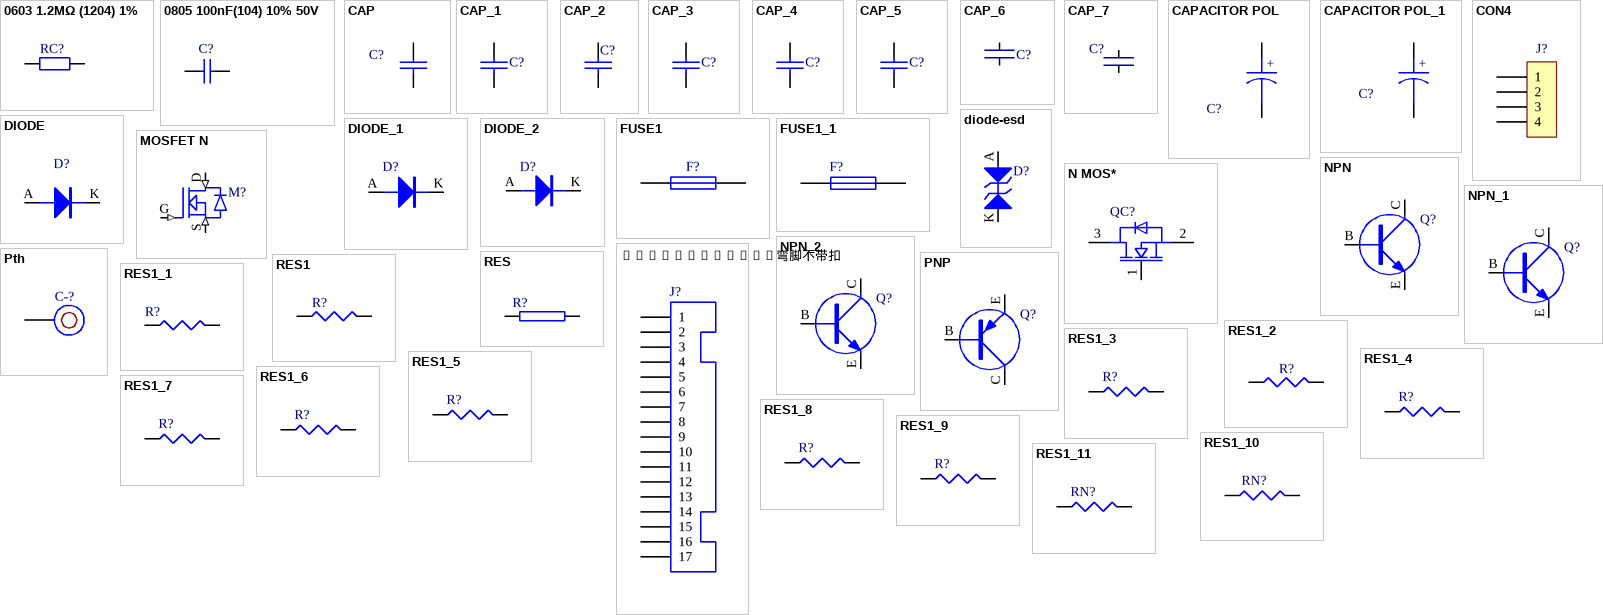
[diagram p0: symbols 0603 1.2MΩ (1204) 1% to RES1_11]
# Altium schematic symbol library MISC86327.SCHLIB: 73 symbols
Pins are listed as number, name and electrical type; pins without a type are passive.


## 0603 1.2MΩ (1204) 1%
designator RC?
chip resistor
footprint RES0603 (CAP0402)
footprint R0603
footprint R0603A (chip resistor)
pins: 1, 2
2 alternate drawings of the same symbol

## 0805 100nF(104) 10% 50V
designator C?
chip capacitor
footprint CAP0603 (CAP0402)
footprint C0603
footprint C0603A (chip capacitor)
pins: 1, 2
2 alternate drawings of the same symbol

## CAP
designator C?
Capacitor
footprint C0603
footprint C0603M (chip capacitor)
pins: 1, 2
2 alternate drawings of the same symbol

## CAP_1
designator C?
Capacitor
footprint C0805
pins: 1, 2
2 alternate drawings of the same symbol

## CAP_2
designator C?
Capacitor
footprint C0603
footprint C0603M (chip capacitor)
pins: 1, 2
2 alternate drawings of the same symbol

## CAP_3
designator C?
Capacitor
footprint C0603
footprint C0805
pins: 1, 2
2 alternate drawings of the same symbol

## CAP_4
designator C?
Capacitor
footprint C0603
footprint C0603M (chip capacitor)
pins: 1, 2
2 alternate drawings of the same symbol

## CAP_5
designator C?
Capacitor
footprint C0603
footprint C0603M (chip capacitor)
pins: 1, 2
2 alternate drawings of the same symbol

## CAP_6
designator C?
CAP
footprint CAP0603 (CAP0402)
footprint C0603
footprint C0603M (chip capacitor)
pins: 1, 2

## CAP_7
designator C?
CAP
footprint CAP0603 (CAP0402)
footprint C0603
footprint C0603M (chip capacitor)
pins: 1, 2

## CAPACITOR POL
designator C?
Capacitor
footprint C0805
pins: 1, 2

## CAPACITOR POL_1
designator C?
Capacitor
footprint C0805
pins: 1, 2

## CON4
designator J?
Connector
footprint CON4/2.0
pins: 1, 2, 3, 4

## DIODE
designator D?
Diode
footprint SOD-323-E
pins: A, K
2 alternate drawings of the same symbol

## diode-esd
designator D?
bidirectional ESD
footprint SMC-BI
pins: A, K

## DIODE_1
designator D?
Diode
footprint SOD-323-E
pins: A, K
2 alternate drawings of the same symbol

## DIODE_2
designator D?
Diode
footprint SOD-323-E
pins: A, K

## FUSE1
designator F?
Fuse
footprint F1206
footprint R1206L (chip resistor)
pins: 1, 2
2 alternate drawings of the same symbol

## FUSE1_1
designator F?
Fuse
footprint F2410
footprint R1206L (chip resistor)
pins: 1, 2
2 alternate drawings of the same symbol

## MOSFET N
designator M?
footprint TOLL
pins: D (in), G (in), S (in)

## N MOS*
designator QC?
chip MOS
footprint TOLL (chip MOS)
footprint TO-252
footprint TO-252-DFN
footprint DFN5X6(T3)
pins: 1 G, 2 S, 3 D

## NPN
designator Q?
NPN Transistor
footprint SOT-23
footprint SOT-23S
pins: B, C, E

## NPN_1
designator Q?
NPN Transistor
footprint SOT-23
footprint SOT-23S
pins: B, C, E
2 alternate drawings of the same symbol

## NPN_2
designator Q?
NPN Transistor
footprint SOT-89BCE
pins: B, C, E

## PH-2.0mm-17P弯脚不带扣
designator J?
PH-2.0mm-17P right-angle connector without latch
footprint PH-2.0mm17P弯脚不带扣 (PH-2.0mm17P right-angle connector without latch)
footprint HY2.0WT-17A/P 卧贴带扣耐温260℃ (horizontal connector)
pins: 1, 2, 3, 4, 5, 6, 7, 8, 9, 10, 11, 12, 13, 14, 15, 16, 17

## PNP
designator Q?
PNP Transistor
footprint SOT-23S
footprint SOT23-3_BEC (chip IC/MOS*)
pins: B, C, E
2 alternate drawings of the same symbol

## Pth
designator C-?
through-hole pad
footprint 4*3 (through-hole pad)
pins: 1

## RES
designator R?
footprint 0603
footprint 0603R
footprint R0603
footprint R0603A (chip resistor)
pins: 1, 2

## RES1
designator R?
footprint R0603
footprint R0603m (chip resistor)
pins: 1, 2

## RES1_1
designator R?
footprint R0603
footprint R0603m (chip resistor)
pins: 1, 2
2 alternate drawings of the same symbol

## RES1_2
designator R?
footprint R0603
footprint R0805
pins: 1, 2
2 alternate drawings of the same symbol

## RES1_3
designator R?
footprint R0603
footprint R0603m (chip resistor)
pins: 1, 2
2 alternate drawings of the same symbol

## RES1_4
designator R?
footprint R0603
footprint R0603m (chip resistor)
pins: 1, 2
2 alternate drawings of the same symbol

## RES1_5
designator R?
footprint R0805
pins: 1, 2
2 alternate drawings of the same symbol

## RES1_6
designator R?
footprint R0603
footprint R0603m (chip resistor)
pins: 1, 2
2 alternate drawings of the same symbol

## RES1_7
designator R?
footprint R0805
pins: 1, 2

## RES1_8
designator R?
footprint R0603
footprint R0603m (chip resistor)
pins: 1, 2

## RES1_9
designator R?
footprint R0603
footprint R0603m (chip resistor)
pins: 1, 2

## RES1_10
designator RN?
footprint R2512A
pins: 1, 2

## RES1_11
designator RN?
footprint R2512A
pins: 1, 2

## RES1_12
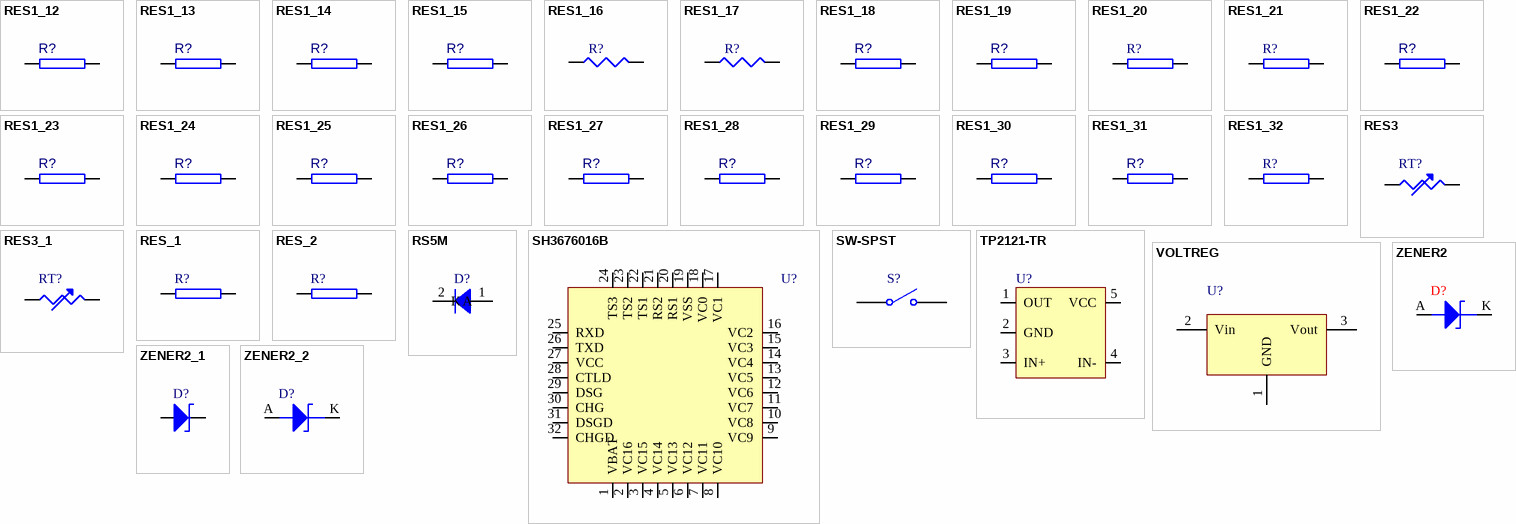
[diagram p1: symbols RES1_12 to ZENER2_2]
## RES1_12
designator R?
RES
footprint AXIAL0.3
footprint AXIAL0.4
footprint AXIAL0.5
footprint AXIAL0.6
footprint 0603
footprint R0603
footprint RES0603 (CAP0402)
footprint RES0603 (CAP0402)
footprint R0603m (chip resistor)
pins: 1, 2
2 alternate drawings of the same symbol

## RES1_13
designator R?
RES
footprint AXIAL0.3
footprint AXIAL0.4
footprint AXIAL0.5
footprint AXIAL0.6
footprint 0603
footprint R0603
footprint RES0603 (CAP0402)
footprint RES0603 (CAP0402)
footprint R0603m (chip resistor)
pins: 1, 2
2 alternate drawings of the same symbol

## RES1_14
designator R?
RES
footprint AXIAL0.3
footprint AXIAL0.4
footprint AXIAL0.5
footprint AXIAL0.6
footprint 0603
footprint R0603
footprint RES0603 (CAP0402)
footprint RES0603 (CAP0402)
footprint R0603m (chip resistor)
pins: 1, 2
2 alternate drawings of the same symbol

## RES1_15
designator R?
RES
footprint AXIAL0.3
footprint AXIAL0.4
footprint AXIAL0.5
footprint AXIAL0.6
footprint 0603
footprint R0603
footprint RES0603 (CAP0402)
footprint RES0603 (CAP0402)
footprint R0603m (chip resistor)
pins: 1, 2
2 alternate drawings of the same symbol

## RES1_16
designator R?
footprint R0805
footprint R0805A (chip resistor)
pins: 1, 2
2 alternate drawings of the same symbol

## RES1_17
designator R?
footprint R0805
footprint R0805A (chip resistor)
pins: 1, 2
2 alternate drawings of the same symbol

## RES1_18
designator R?
RES
footprint AXIAL0.3
footprint AXIAL0.4
footprint AXIAL0.5
footprint AXIAL0.6
footprint AXIAL0.8
footprint AXIAL0.8-2
footprint AXIAL1.2
footprint AXIAL1.2-2
footprint 0402
footprint 0603
footprint 0805
footprint RES0603 (CAP0402)
footprint R0603
footprint R0603A (chip resistor)
pins: 1, 2

## RES1_19
designator R?
RES
footprint AXIAL0.3
footprint AXIAL0.4
footprint AXIAL0.5
footprint AXIAL0.6
footprint AXIAL0.8
footprint AXIAL0.8-2
footprint AXIAL1.2
footprint AXIAL1.2-2
footprint 0402
footprint 0603
footprint 0805
footprint RES0603 (CAP0402)
footprint R0603
footprint R0603A (chip resistor)
pins: 1, 2

## RES1_20
designator R?
RES
footprint 0603
footprint RES0603 (CAP0402)
footprint R0603
footprint R0603A (chip resistor)
pins: 1, 2

## RES1_21
designator R?
RES
footprint 0603
footprint RES0603 (CAP0402)
footprint R0603
footprint R0603A (chip resistor)
pins: 1, 2

## RES1_22
designator R?
RES
footprint AXIAL0.3
footprint AXIAL0.4
footprint AXIAL0.5
footprint AXIAL0.6
footprint AXIAL0.8
footprint AXIAL0.8-2
footprint AXIAL1.2
footprint AXIAL1.2-2
footprint 0402
footprint 0603
footprint 0805
footprint RES0603 (CAP0402)
footprint R0603
footprint R0603A (chip resistor)
pins: 1, 2

## RES1_23
designator R?
RES
footprint AXIAL0.3
footprint AXIAL0.4
footprint AXIAL0.5
footprint AXIAL0.6
footprint AXIAL0.8
footprint AXIAL0.8-2
footprint AXIAL1.2
footprint AXIAL1.2-2
footprint 0402
footprint 0603
footprint 0805
footprint RES0603 (CAP0402)
footprint R0603
footprint R0603A (chip resistor)
pins: 1, 2

## RES1_24
designator R?
RES
footprint AXIAL0.3
footprint AXIAL0.4
footprint AXIAL0.5
footprint AXIAL0.6
footprint AXIAL0.8
footprint AXIAL0.8-2
footprint AXIAL1.2
footprint AXIAL1.2-2
footprint 0402
footprint 0603
footprint 0805
footprint RES0603 (CAP0402)
footprint R0603
footprint R0603A (chip resistor)
pins: 1, 2

## RES1_25
designator R?
RES
footprint AXIAL0.3
footprint AXIAL0.4
footprint AXIAL0.5
footprint AXIAL0.6
footprint AXIAL0.8
footprint AXIAL0.8-2
footprint AXIAL1.2
footprint AXIAL1.2-2
footprint 0402
footprint 0603
footprint 0805
footprint RES0603 (CAP0402)
footprint R0603
footprint R0603A (chip resistor)
pins: 1, 2

## RES1_26
designator R?
RES
footprint AXIAL0.3
footprint AXIAL0.4
footprint AXIAL0.5
footprint AXIAL0.6
footprint AXIAL0.8
footprint AXIAL0.8-2
footprint AXIAL1.2
footprint AXIAL1.2-2
footprint 0402
footprint 0603
footprint 0805
footprint RES0603 (CAP0402)
footprint R0603
footprint R0603A (chip resistor)
pins: 1, 2

## RES1_27
designator R?
RES
footprint AXIAL0.3
footprint AXIAL0.4
footprint AXIAL0.5
footprint AXIAL0.6
footprint AXIAL0.8
footprint AXIAL0.8-2
footprint AXIAL1.2
footprint AXIAL1.2-2
footprint 0402
footprint 0603
footprint 0805
footprint RES0603 (CAP0402)
footprint R0603
footprint R0603A (chip resistor)
pins: 1, 2

## RES1_28
designator R?
RES
footprint AXIAL0.3
footprint AXIAL0.4
footprint AXIAL0.5
footprint AXIAL0.6
footprint AXIAL0.8
footprint AXIAL0.8-2
footprint AXIAL1.2
footprint AXIAL1.2-2
footprint 0402
footprint 0603
footprint 0805
footprint RES0603 (CAP0402)
footprint R0603
footprint R0603A (chip resistor)
pins: 1, 2

## RES1_29
designator R?
RES
footprint AXIAL0.3
footprint AXIAL0.4
footprint AXIAL0.5
footprint AXIAL0.6
footprint AXIAL0.8
footprint AXIAL0.8-2
footprint AXIAL1.2
footprint AXIAL1.2-2
footprint 0402
footprint 0603
footprint 0805
footprint RES0603 (CAP0402)
footprint R0603
footprint R0603A (chip resistor)
pins: 1, 2

## RES1_30
designator R?
RES
footprint AXIAL0.3
footprint AXIAL0.4
footprint AXIAL0.5
footprint AXIAL0.6
footprint AXIAL0.8
footprint AXIAL0.8-2
footprint AXIAL1.2
footprint AXIAL1.2-2
footprint 0402
footprint 0603
footprint 0805
footprint RES0603 (CAP0402)
footprint R0603
footprint R0603A (chip resistor)
pins: 1, 2

## RES1_31
designator R?
RES
footprint AXIAL0.3
footprint AXIAL0.4
footprint AXIAL0.5
footprint AXIAL0.6
footprint AXIAL0.8
footprint AXIAL0.8-2
footprint AXIAL1.2
footprint AXIAL1.2-2
footprint 0402
footprint 0603
footprint 0805
footprint RES0603 (CAP0402)
footprint R0603
footprint R0603A (chip resistor)
pins: 1, 2

## RES1_32
designator R?
RES
footprint 0603
footprint RES0603 (CAP0402)
footprint R0603
footprint R0603A (chip resistor)
pins: 1, 2

## RES3
designator RT?
footprint NTC-DIP
pins: 1, 2
2 alternate drawings of the same symbol

## RES3_1
designator RT?
footprint NTC-DIP
footprint R0603
pins: 1, 2
2 alternate drawings of the same symbol

## RES_1
designator R?
footprint 0603
footprint 0603R
footprint R0603
footprint R0603A (chip resistor)
pins: 1, 2

## RES_2
designator R?
footprint 0603
footprint 0603R
footprint R0603
footprint R0603A (chip resistor)
pins: 1, 2

## RS5M
designator D?
chip diode
footprint SMAF
footprint SMB(DO-214AA) (chip diode)
footprint SMC A(DO-214AB) (chip diode)
footprint SMC A(DO-214AB) (chip diode)
footprint SMC_MDO-214AB) (chip diode)
pins: 1 K, 2 A

## SH3676016B
designator U?
footprint LQFP-32
pins: 1 VBAT, 2 VC16, 3 VC15, 4 VC14, 5 VC13, 6 VC12, 7 VC11, 8 VC10, 9 VC9, 10 VC8, 11 VC7, 12 VC6, 13 VC5, 14 VC4, 15 VC3, 16 VC2, 17 VC1, 18 VC0, 19 VSS, 20 RS1, 21 RS2, 22 TS1, 23 TS2, 24 TS3, 25 RXD, 26 TXD, 27 VCC, 28 CTLD, 29 DSG, 30 CHG, 31 DSGD, 32 CHGD

## SW-SPST
designator S?
Single-Pole, Single-Throw Switch
footprint WK
footprint NTC-DIP
footprint RT2.3X1.2-2 (NTC with wire leads)
footprint NTC-DIP
pins: 1 COMMON, 2 NO

## TP2121-TR
designator U?
S8211D
footprint SOT23-5
pins: 1 OUT, 2 GND, 3 IN+, 4 IN-, 5 VCC
2 alternate drawings of the same symbol

## VOLTREG
designator U?
footprint TO220H
footprint SO-89
pins: 1 GND, 2 Vin, 3 Vout

## ZENER2
designator D?
Zener Diode
footprint SOD-323-E
footprint SMA
pins: A, K
2 alternate drawings of the same symbol

## ZENER2_1
designator D?
Zener Diode
footprint SOD-323-E
pins: A, K

## ZENER2_2
designator D?
Zener Diode
footprint SOD-323-E
footprint SOD323(1+2-) (chip diode)
footprint SOD323(A+K-) (chip diode)
pins: A, K